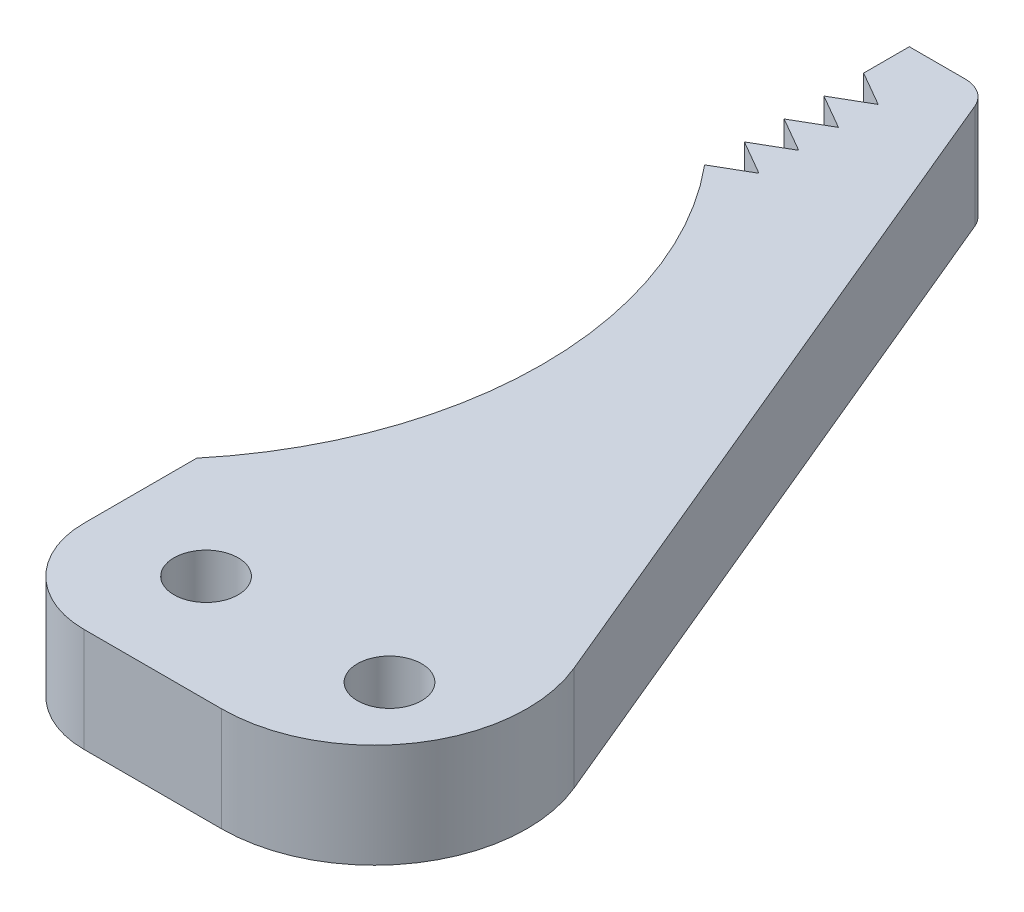
SolidWorks part; units mm, degrees
ref_plane "Front Plane" through (0, 0, 0) normal (0, 0, 1) x (1, 0, 0)
ref_plane "Top Plane" through (0, 0, 0) normal (0, 1, 0) x (1, 0, 0)
ref_plane "Right Plane" through (0, 0, 0) normal (1, 0, 0) x (0, 0, -1)
sketch "Sketch1" plane through (0, 0, 0) normal (0, 1, 0) x (1, 0, 0)
  line L0 (0, 0) -> (38.1, 0)
  line L1 (38.1, 0) -> (6.35, 76.2)
  line L2 (6.35, 76.2) -> (0, 76.2)
  line L3 (0, 76.2) -> (0, 59.1988)
  line L4 (0, 0) -> (0, 17.0012)
  arc A0 (0, 17.0012) -> (0, 59.1988) centre (-25.4, 38.1) ccw
  dimension "D3" = 25.4
  dimension "D4" = 38.1
  dimension "D5" = 33.02
  dimension "D1" = 38.1
  dimension "D2" = 6.35
  dimension "D6" = 76.2
extrude "Boss-Extrude1" add sketch "Sketch1" along normal blind 8.636
sketch "Sketch3" plane through (0, 8.636, 0) normal (0, 1, 0) x (1, 0, 0)
  line L0 (0, 0) -> (38.1, 0) construction
  line L2 (0, 17.0012) -> (0, 0) construction
  circle A0 centre (8.89, 8.89) radius 2.667
  circle A1 centre (24.13, 8.89) radius 2.667
  dimension "D1" = 5.334
  dimension "D2" = 5.334
  dimension "D3" = 8.89
  dimension "D4" = 8.89
  dimension "D5" = 8.89
  dimension "D6" = 15.24
extrude "Cut-Extrude1" cut sketch "Sketch3" against normal blind 19.05
fillet "Fillet1" radius 12.7 1 edges at (38.1, 4.318, 0)
fillet "Fillet2" radius 2.54 1 edges at (6.35, 4.318, -76.2)
fillet "Fillet3" radius 7.62 1 edges at (0, 4.318, 0)
sketch "Sketch4" plane through (0, 8.636, 0) normal (0, 1, 0) x (1, 0, 0)
  line L0 (0, 59.1988) -> (2.8596, 60.8498)
  line L1 (2.8596, 60.8498) -> (0, 62.5008)
  line L2 (0, 76.2) -> (0, 59.1988) construction
  line L3 (0, 59.1988) -> (0, 62.5008)
  line L4 (0, 62.5008) -> (-0.0033, 62.4368)
  line L5 (0, 62.5008) -> (2.8596, 64.1518)
  line L6 (2.8596, 64.1518) -> (0, 65.8028)
  line L7 (0, 62.5008) -> (0, 65.8028)
  line L8 (0, 65.8028) -> (-0.0033, 65.7388)
  line L9 (0, 65.8028) -> (2.8596, 67.4538)
  line L10 (2.8596, 67.4538) -> (0, 69.1048)
  line L11 (0, 65.8028) -> (0, 69.1048)
  line L12 (0, 69.1048) -> (-0.0033, 69.0408)
  line L13 (0, 69.1048) -> (2.8596, 70.7558)
  line L14 (2.8596, 70.7558) -> (0, 72.4068)
  line L15 (0, 69.1048) -> (0, 72.4068)
  line L16 (0, 72.4068) -> (-0.0033, 72.3428)
  line M10 (0, 76.2) -> (0, 59.1988)
  dimension "D1" = 60
  dimension "D2" = 3.302
  dimension "D3" = 3.302
  dimension "D4" = 4
extrude "Cut-Extrude2" cut sketch "Sketch4" against normal through all contours L0 L1 M10 | L5 L6 M10 | L9 L10 M10 | L13 L14 M10
scale "Scale1" bodies to scale 103 scale about origin uniform scaling yes scale factor 2
